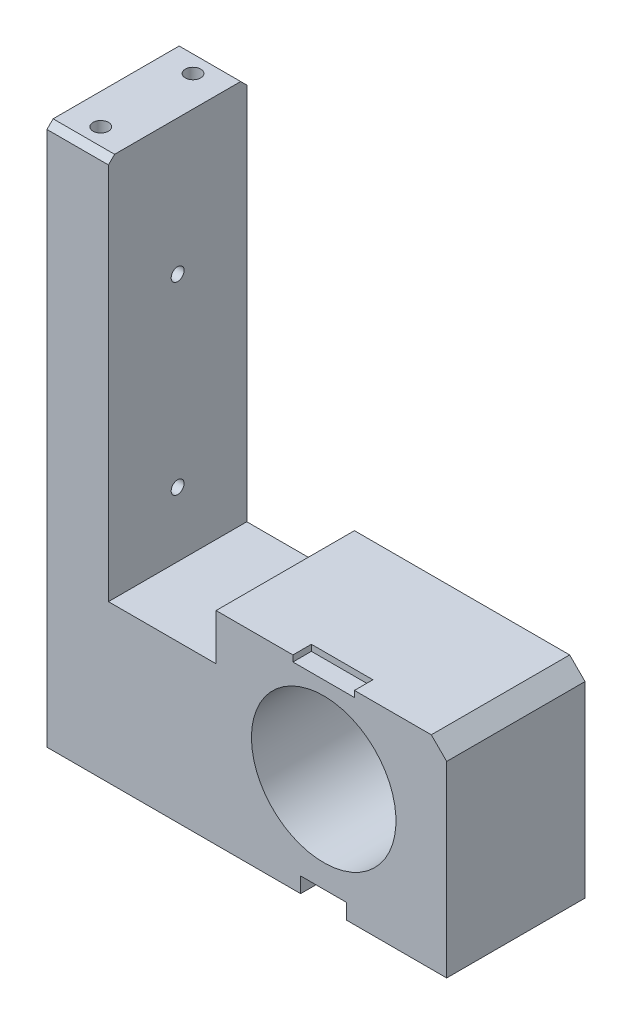
SolidWorks part; units mm, degrees
ref_plane "Front Plane" through (0, 0, 0) normal (0, 0, 1) x (1, 0, 0)
ref_plane "Top Plane" through (0, 0, 0) normal (0, 1, 0) x (1, 0, 0)
ref_plane "Right Plane" through (0, 0, 0) normal (1, 0, 0) x (0, 0, -1)
sketch "Sketch1" plane through (0, 0, 0) normal (0, 0, 1) x (1, 0, 0)
  line L0 (-90, 140) -> (-90, -36)
  line L1 (-90, -36) -> (-7.5, -36)
  line L2 (7.5, -36) -> (40, -36)
  line L4 (40, -36) -> (40, 30)
  line L5 (-70, 140) -> (-70, 30)
  line L6 (-70, 30) -> (40, 30)
  line L7 (-90, 140) -> (-70, 140)
  line L8 (-7.5, -36) -> (-7.5, -31)
  line L9 (-7.5, -31) -> (7.5, -31)
  line L10 (7.5, -36) -> (7.5, -31)
  circle A0 centre (0, 0) radius 23.5
  dimension "D1" = 47
  dimension "D3" = 30
  dimension "D2" = 130
  dimension "D4" = 40
  dimension "D5" = 176
  dimension "D6" = 66
  dimension "D7" = 20
  dimension "D8" = 15
  dimension "D9" = 32.5
  dimension "D10" = 5
extrude "Boss-Extrude1" add sketch "Sketch1" along normal blind 45
hole_wizard "M6 Tapped Hole1" positions "Sketch3" profile "Sketch2" tap size "M6" standard "Gb"
sketch "Sketch3" plane through (0, -36, 0) normal (0, -1, 0) x (1, 0, 0)
  line L0 (-90, 0) -> (-7.5, 0) construction
  line L3 (40, 45) -> (40, 0) construction
  point P0 (-75, 10)
  point P3 (25, 10)
  point P10 (-75, 35)
  point P12 (25, 35)
  dimension "D1" = 10
  dimension "D2" = 100
  dimension "D3" = 15
  dimension "D5" = 25
sketch "Sketch2" plane through (-75, -36, 10) normal (1, 0, 0) x (0, 0, -1)
  line L0 (0, 0) -> (0, 16.5022)
  line L1 (0, 16.5022) -> (2.5, 15)
  line L2 (2.5, 15) -> (2.5, 0)
  line L5 (2.5, 0) -> (0, 0)
  line L10 (0, 16.5022) -> (-2.5, 15) construction
  line L11 (0, -6.35) -> (0, 107.95) construction
  dimension "螺纹孔钻头直径" = 5
  dimension "螺纹孔钻头深度" = 15
  dimension "导头角度" = 118
cosmetic thread "Cosmetic Thread2" parameters "D1"=12, "D2"=6
cosmetic thread "Cosmetic Thread3" parameters "D1"=12, "D2"=6
cosmetic thread "Cosmetic Thread4" parameters "D1"=12, "D2"=6
cosmetic thread "Cosmetic Thread12" parameters "D1"=12, "D2"=6
hole_wizard "M5 Tapped Hole1" positions "Sketch7" profile "Sketch6" tap size "M5" standard "GB" end condition through all
sketch "Sketch7" plane through (-70, 0, 0) normal (1, 0, 0) x (0, 0, -1)
  line L0 (-45, 140) -> (0, 140) construction
  line L1 (-45, 30) -> (-45, 140) construction
  point P0 (-22.5, 96)
  point P1 (-22.5, 36)
  dimension "D1" = 60
  dimension "D2" = 44
  dimension "D3" = 22.5
cosmetic thread "Cosmetic Thread7" parameters "D2"=5
cosmetic thread "Cosmetic Thread8" parameters "D2"=5
sketch "Sketch6" plane through (-70, 96, 22.5) normal (0, 1, 0) x (0, 0, -1)
  line L0 (0, 0) -> (0, 20)
  line L1 (0, 20) -> (2.1, 20)
  line L2 (2.1, 20) -> (2.1, 0)
  line L5 (2.1, 0) -> (0, 0)
  line L11 (0, -6.35) -> (0, 107.95) construction
  dimension "通孔螺纹孔钻头直径" = 4.2
  dimension "通孔螺纹孔钻头深度" = 20
hole_wizard "M6 Tapped Hole2" positions "Sketch9" profile "Sketch8" tap size "M6" standard "GB"
sketch "Sketch9" plane through (0, 140, 0) normal (0, 1, 0) x (-1, 0, 0)
  line L0 (70, 0) -> (90, 0) construction
  line L1 (90, 45) -> (90, 0) construction
  point P0 (80, 7.5)
  point P1 (80, 37.5)
  dimension "D1" = 30
  dimension "D2" = 7.5
  dimension "D3" = 10
sketch "Sketch8" plane through (-80, 140, 7.5) normal (1, 0, 0) x (0, 0, 1)
  line L0 (0, 0) -> (0, 16.5022)
  line L1 (0, 16.5022) -> (2.5, 15)
  line L2 (2.5, 15) -> (2.5, 0)
  line L5 (2.5, 0) -> (0, 0)
  line L10 (0, 16.5022) -> (-2.5, 15) construction
  line L11 (0, -6.35) -> (0, 107.95) construction
  dimension "螺纹孔钻头直径" = 5
  dimension "螺纹孔钻头深度" = 15
  dimension "导头角度" = 118
cosmetic thread "Cosmetic Thread9" parameters "D1"=12, "D2"=6
cosmetic thread "Cosmetic Thread10" parameters "D1"=12, "D2"=6
hole_wizard "M4 Tapped Hole1" positions "Sketch11" profile "Sketch10" tap size "M4" standard "GB"
sketch "Sketch11" plane through (0, 0, 0) normal (0, 0, -1) x (-1, 0, 0)
  line L0 (0, 27.5) -> (0, -27.5) construction
  line L1 (-19.4454, -19.4454) -> (19.4454, 19.4454) construction
  line L2 (-19.4454, 19.4454) -> (19.4454, -19.4454) construction
  circle A0 centre (0, 0) radius 27.5 construction
  point P0 (-19.4454, 19.4454)
  point P1 (19.4454, -19.4454)
  point P3 (-19.4454, -19.4454)
  point P5 (19.4454, 19.4454)
  dimension "D3" = 55
  dimension "D1" = 45
  dimension "D2" = 45
sketch "Sketch10" plane through (19.4454, 19.4454, 0) normal (1, 0, 0) x (0, 1, 0)
  line L0 (0, 0) -> (0, 11.0914)
  line L1 (0, 11.0914) -> (1.65, 10.1)
  line L2 (1.65, 10.1) -> (1.65, 0)
  line L5 (1.65, 0) -> (0, 0)
  line L10 (0, 11.0914) -> (-1.65, 10.1) construction
  line L11 (0, -6.35) -> (0, 107.95) construction
  dimension "螺纹孔钻头直径" = 3.3
  dimension "螺纹孔钻头深度" = 10.1
  dimension "导头角度" = 118
cosmetic thread "Cosmetic Thread13" parameters "D1"=8, "D2"=4
cosmetic thread "Cosmetic Thread14" parameters "D1"=8, "D2"=4
cosmetic thread "Cosmetic Thread15" parameters "D1"=8, "D2"=4
cosmetic thread "Cosmetic Thread16" parameters "D1"=8, "D2"=4
chamfer "Chamfer1" distance 5 angle 45 1 edges at (40, 30, 22.5)
chamfer "Chamfer2" distance 2 angle 45 2 edges at (-80, 140, 45) (-80, 140, 0)
sketch "Sketch18" plane through (0, 0, 0) normal (0, 0, -1) x (-1, 0, 0)
  line L1 (70, 30) -> (35, 30)
  line L2 (70, 30) -> (70, 15)
  line L3 (70, 15) -> (35, 15)
  line L4 (35, 30) -> (35, 15)
  dimension "D1" = 35
  dimension "D2" = 15
extrude "Cut-Extrude1" cut sketch "Sketch18" against normal through all
sketch "Sketch19" plane through (0, 30, 0) normal (0, 1, 0) x (1, 0, 0)
  line L0 (35, -45) -> (-35, -45) construction
  line L1 (-10, -45) -> (10, -45)
  line L2 (-10, -45) -> (-10, -39)
  line L3 (-10, -39) -> (10, -39)
  line L4 (10, -45) -> (10, -39)
  line L5 (0, 0) -> (0, -63.9596) construction
  dimension "D1" = 20
  dimension "D2" = 6
extrude "Cut-Extrude2" cut sketch "Sketch19" against normal blind 2
